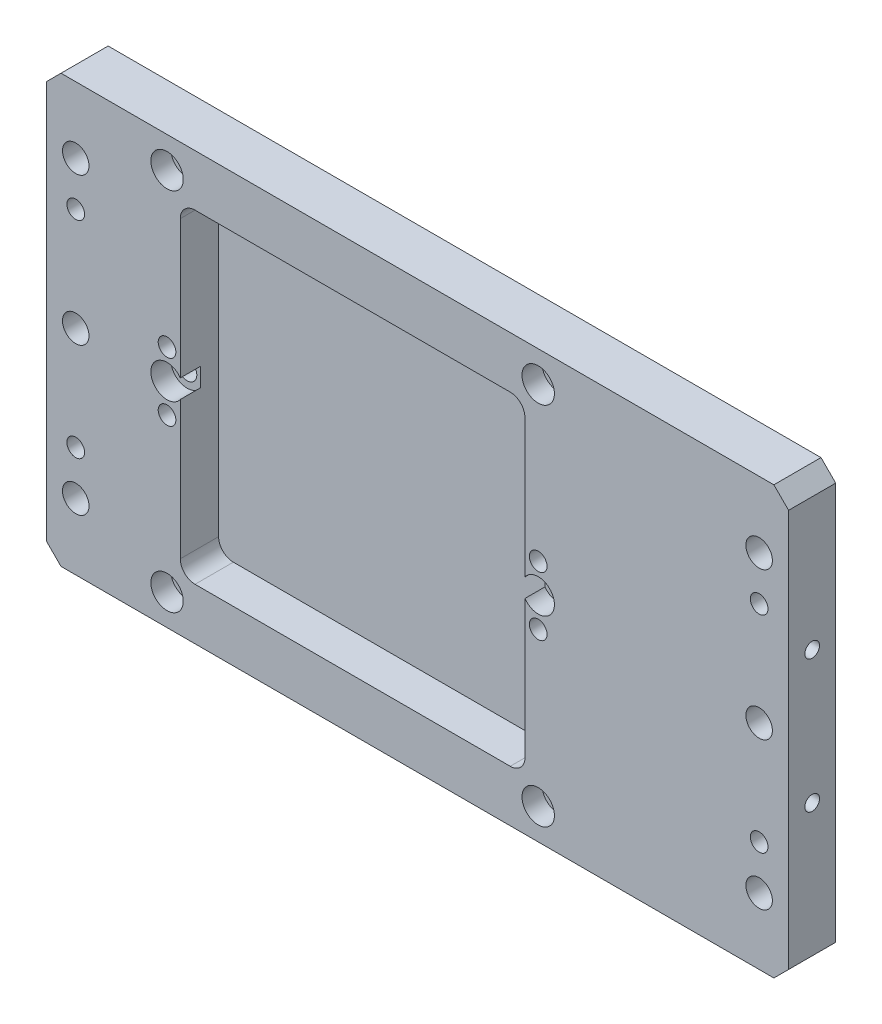
from build123d import *

# Parameters (mm, degrees)
SKETCH_1_W                  = 252
SKETCH_1_H                  = 145
EXTRUDE_1_DEPTH             = 8
HOLE_WIZARD_2_D             = 6.6
HOLE_WIZARD_2_CBORE_D       = 11
HOLE_WIZARD_2_CBORE_DEPTH   = 6.8
HOLE_WIZARD_2_2_D           = 9
HOLE_WIZARD_2_2_CBORE_D     = 15
HOLE_WIZARD_2_2_CBORE_DEPTH = 9
HOLE_WIZARD_6_0_6_1_D       = 6
HOLE_WIZARD_6_0_6_2_D       = 6
CUT_EXTRUDE_1_DEPTH         = 13
CHAMFER_1_SIZE              = 5
HOLE_WIZARD_M6_2_D          = 5
HOLE_WIZARD_M6_2_DEPTH      = 23
HOLE_WIZARD_M6_2_TIP        = 1.502151548


with BuildPart() as part:
    # 草图1 → 凸台-拉伸1 (new, symmetric)
    with BuildSketch(Plane.XY):
        Rectangle(SKETCH_1_W, SKETCH_1_H)
    extrude(amount=EXTRUDE_1_DEPTH, both=True)

    # Hole Wizard 2 (through all)
    with Locations(Plane.XY.offset(8)):
        with Locations((-85, 62), (-85, 0), (41, 62), (41, 0), (41, -62), (-85, -62)):
            CounterBoreHole(HOLE_WIZARD_2_D / 2, HOLE_WIZARD_2_CBORE_D / 2, HOLE_WIZARD_2_CBORE_DEPTH)

    # Hole Wizard 2 2 (through all)
    with Locations(Plane(origin=(0, 0, -8), x_dir=(-1, 0, 0), z_dir=(0, 0, -1))):
        with Locations((-116, -50), (-116, 0), (-116, 50)):
            hole_wizard_2_2 = CounterBoreHole(HOLE_WIZARD_2_2_D / 2, HOLE_WIZARD_2_2_CBORE_D / 2, HOLE_WIZARD_2_2_CBORE_DEPTH)

    # Ø6.0 (6) 直径孔1 (through all)
    with Locations(Plane(origin=(0, 0, -8), x_dir=(-1, 0, 0), z_dir=(0, 0, -1))):
        with Locations((-116, -35), (-116, 35)):
            hole_wizard_6_0_6_1 = Hole(HOLE_WIZARD_6_0_6_1_D / 2)

    # 镜向1: Hole Wizard 2 2, Ø6.0 (6) 直径孔1 across plane
    add(hole_wizard_2_2.mirror(Plane(origin=(0, 0, 0), x_dir=(0, 0, 1), z_dir=(1, 0, 0))), mode=Mode.SUBTRACT)
    add(hole_wizard_6_0_6_1.mirror(Plane(origin=(0, 0, 0), x_dir=(0, 0, 1), z_dir=(1, 0, 0))), mode=Mode.SUBTRACT)

    # Ø6.0 (6) 直径孔2 (through all)
    with Locations(Plane.XY.offset(8)):
        with Locations((41, -10), (-85, -10), (-85, 10), (41, 10)):
            Hole(HOLE_WIZARD_6_0_6_2_D / 2)

    # 草图10 → 切除-拉伸1 (cut)
    with BuildSketch(Plane.XY.offset(8)):
        with BuildLine():
            Line((-75.5, 55), (31.5, 55))
            ThreePointArc((31.5, 55), (35.035533906, 53.535533906), (36.5, 50))
            Line((36.5, 50), (36.5, -50))
            ThreePointArc((36.5, -50), (35.035533906, -53.535533906), (31.5, -55))
            Line((31.5, -55), (-75.5, -55))
            ThreePointArc((-75.5, -55), (-79.035533906, -53.535533906), (-80.5, -50))
            Line((-80.5, -50), (-80.5, 50))
            ThreePointArc((-80.5, 50), (-79.035533906, 53.535533906), (-75.5, 55))
        make_face()
    extrude(amount=-CUT_EXTRUDE_1_DEPTH, mode=Mode.SUBTRACT)

    # 倒角1
    chamfer_1_edges = [part.edges().sort_by_distance(p)[0] for p in [
        (-126, 72.5, 0),
        (126, 72.5, 0),
        (126, -72.5, 0),
        (-126, -72.5, 0),
    ]]
    chamfer(chamfer_1_edges, length=CHAMFER_1_SIZE)

    # M6 螺纹孔2
    with Locations(Plane(origin=(126, 0, 0), x_dir=(0, 0, -1), z_dir=(1, 0, 0))):
        with Locations((0, 22.5), (0, -22.5)):
            Hole(HOLE_WIZARD_M6_2_D / 2, depth=HOLE_WIZARD_M6_2_DEPTH)
            with Locations((0, 0, -(HOLE_WIZARD_M6_2_DEPTH + HOLE_WIZARD_M6_2_TIP / 2))):  # 118° drill point
                Cone(0, HOLE_WIZARD_M6_2_D / 2, HOLE_WIZARD_M6_2_TIP, mode=Mode.SUBTRACT)


solid = part.part
